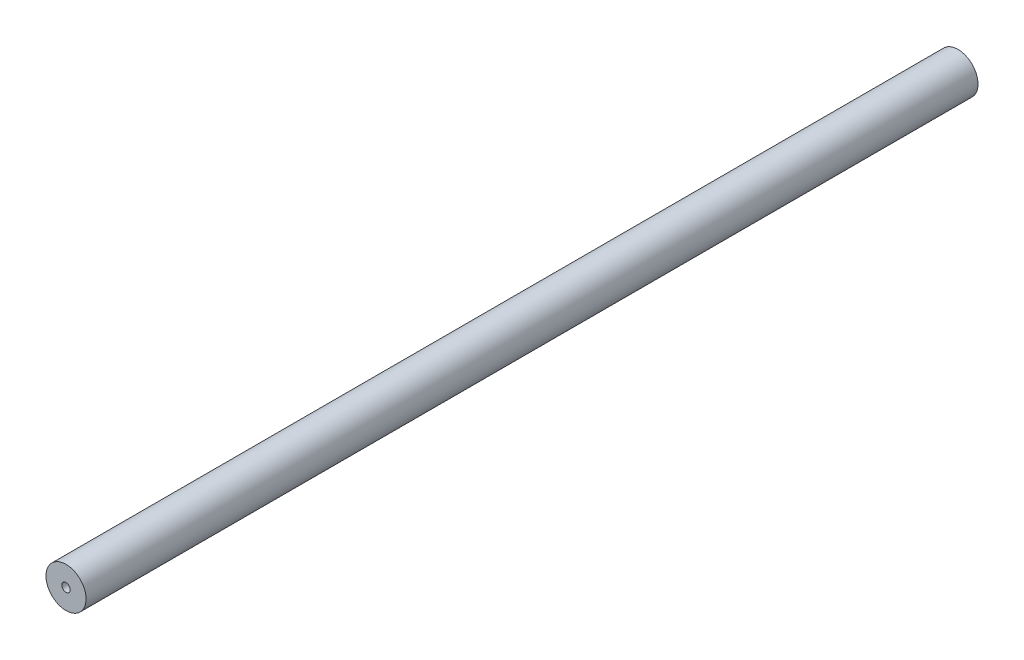
SolidWorks part; units mm, degrees
ref_plane "前视基准面" through (0, 0, 0) normal (0, 0, 1) x (1, 0, 0)
ref_plane "上视基准面" through (0, 0, 0) normal (0, 1, 0) x (1, 0, 0)
ref_plane "右视基准面" through (0, 0, 0) normal (1, 0, 0) x (0, 0, -1)
sketch "草图1" plane through (0, 0, 0) normal (0, 0, 1) x (1, 0, 0)
  circle A0 centre (0, 0) radius 10
  dimension "D1" = 20
extrude "凸台-拉伸1" add sketch "草图1" along normal blind 445
hole_wizard "M5 螺纹孔1" positions "草图3" profile "草图2" tap size "M5" standard "Iso"
sketch "草图3" plane through (0, 0, 445) normal (0, 0, 1) x (1, 0, 0)
  point P0 (0, 0)
sketch "草图2" plane through (0, 0, 445) normal (1, 0, 0) x (0, -1, 0)
  line L0 (0, 0) -> (0, 16.2618)
  line L1 (0, 16.2618) -> (2.1, 15)
  line L2 (2.1, 15) -> (2.1, 0)
  line L5 (2.1, 0) -> (0, 0)
  line L10 (0, 16.2618) -> (-2.1, 15) construction
  line L11 (0, -6.35) -> (0, 107.95) construction
  dimension "螺纹孔钻头直径" = 4.2
  dimension "螺纹孔钻头深度" = 15
  dimension "导头角度" = 118
cosmetic thread "孔螺蚊线1" parameters "D1"=13, "D2"=5
hole_wizard "M5 螺纹孔2" positions "草图5" profile "草图4" tap size "M5" standard "Iso"
sketch "草图5" plane through (0, 0, 0) normal (0, 0, -1) x (-1, 0, 0)
  point P0 (0, 0)
sketch "草图4" plane through (0, 0, 0) normal (1, 0, 0) x (0, 1, 0)
  line L0 (0, 0) -> (0, 16.2618)
  line L1 (0, 16.2618) -> (2.1, 15)
  line L2 (2.1, 15) -> (2.1, 0)
  line L5 (2.1, 0) -> (0, 0)
  line L10 (0, 16.2618) -> (-2.1, 15) construction
  line L11 (0, -6.35) -> (0, 107.95) construction
  dimension "螺纹孔钻头直径" = 4.2
  dimension "螺纹孔钻头深度" = 15
  dimension "导头角度" = 118
cosmetic thread "孔螺蚊线2" parameters "D1"=13, "D2"=5
